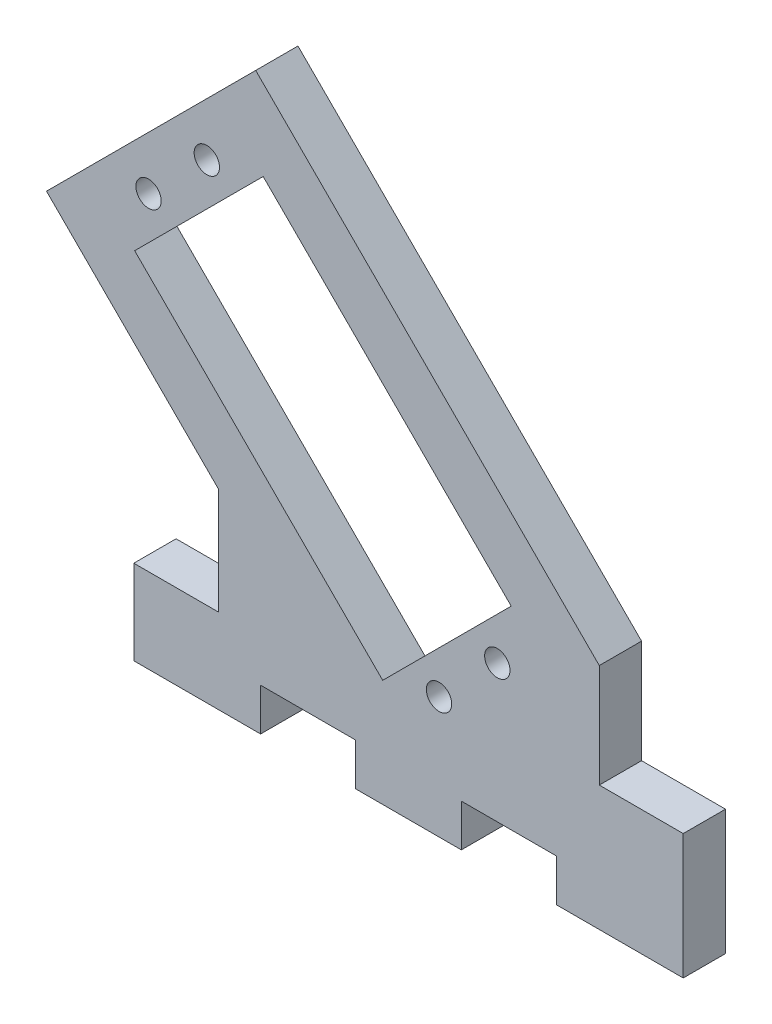
from build123d import *

# Parameters (mm, degrees)
SKETCH_1_R      = 1.5
EXTRUDE_1_DEPTH = 5


with BuildPart() as part:
    # 草图1 → 凸台-拉伸1 (new body)
    with BuildSketch(Plane.XY):
        Polygon((-12.648598414, -34.707783696), (-27.648598414, -34.707783696), (-27.648598414, -24.707783696), (-17.648598414, -24.707783696), (-17.648598414, -12.085840997), (-37.977918373, 8.243478962), (-13.229181032, 32.992216304), (27.420818968, -7.657783696), (27.420818968, -19.907783696), (37.351401586, -19.907783696), (37.351401586, -34.707783696), (22.351401586, -34.707783696), (22.351401586, -29.707783696), (11.101401586, -29.707783696), (11.101401586, -34.707783696), (-1.398598414, -34.707783696), (-1.398598414, -29.707783696), (-12.648598414, -29.707783696), align=None)
        with Locations((-19.009778968, 20.918368015)):
            Circle(SKETCH_1_R, mode=Mode.SUBTRACT)
        with Locations((-25.904070084, 14.024076898)):
            Circle(SKETCH_1_R, mode=Mode.SUBTRACT)
        with Locations((15.355610598, -13.447021551)):
            Circle(SKETCH_1_R, mode=Mode.SUBTRACT)
        with Locations((8.461319481, -20.341312667)):
            Circle(SKETCH_1_R, mode=Mode.SUBTRACT)
        Polygon((-27.548093351, 7.359595486), (1.796838069, -21.985335933), (16.999633864, -6.782540138), (-12.345297555, 22.562391281), align=None, mode=Mode.SUBTRACT)
    extrude(amount=EXTRUDE_1_DEPTH)


solid = part.part
